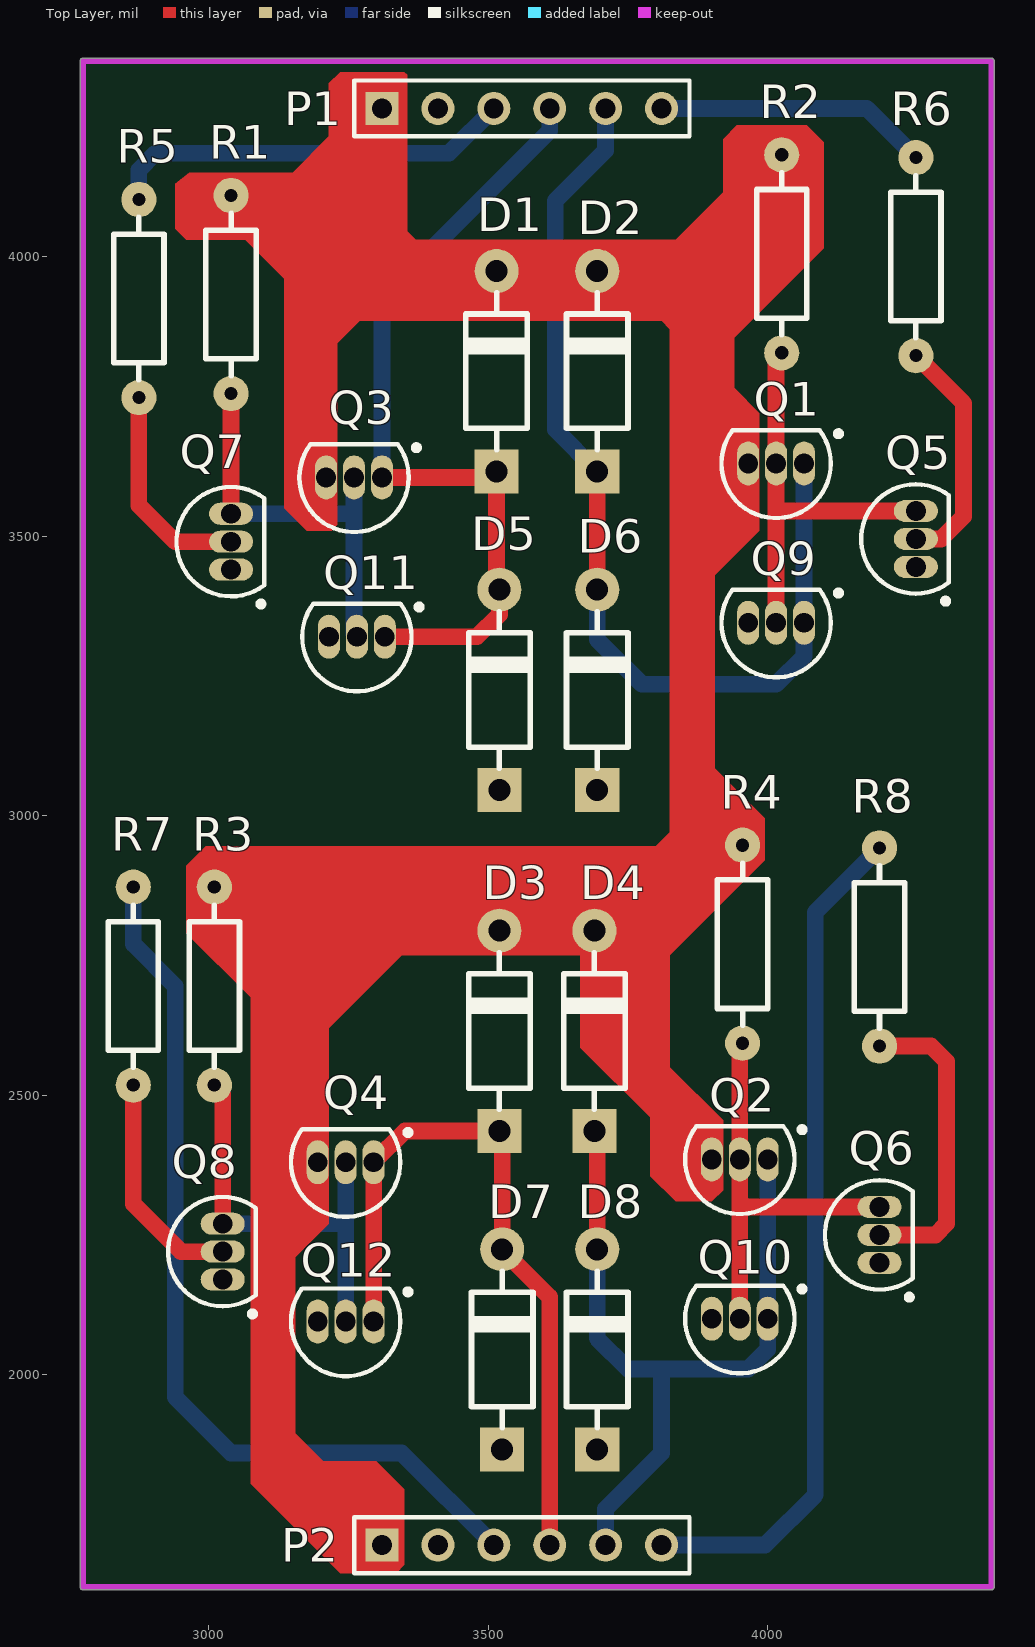
[diagram p0: Top Layer view]
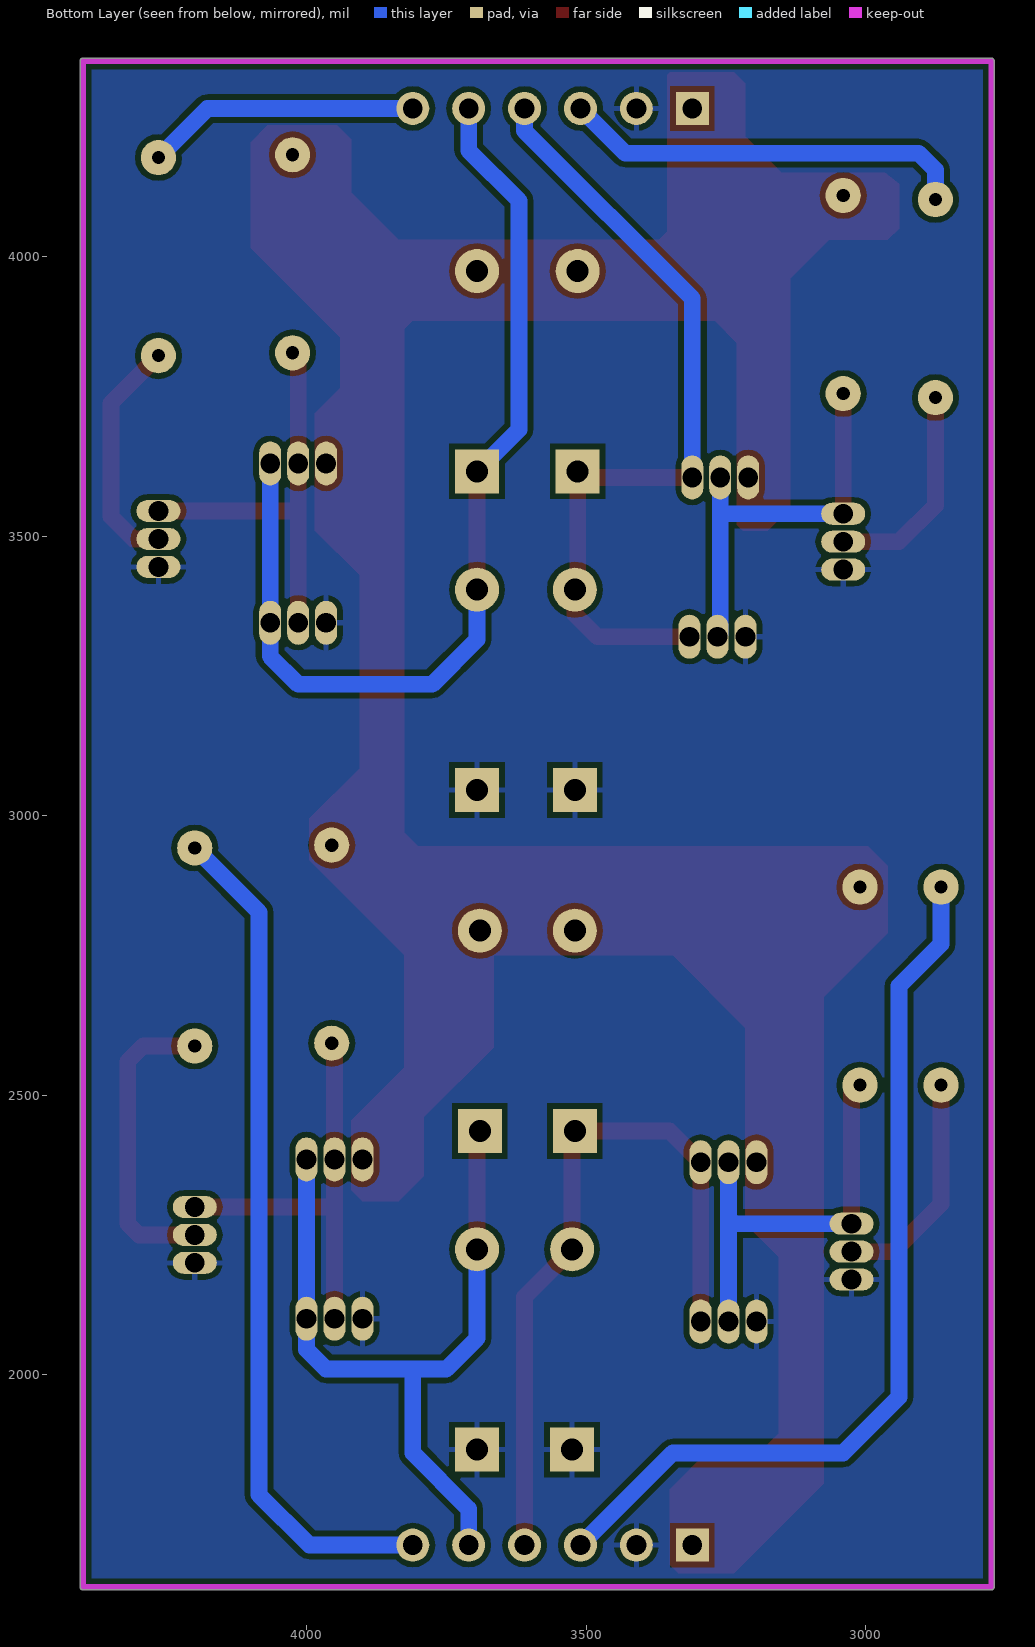
[diagram p1: Bottom Layer view, seen from below]
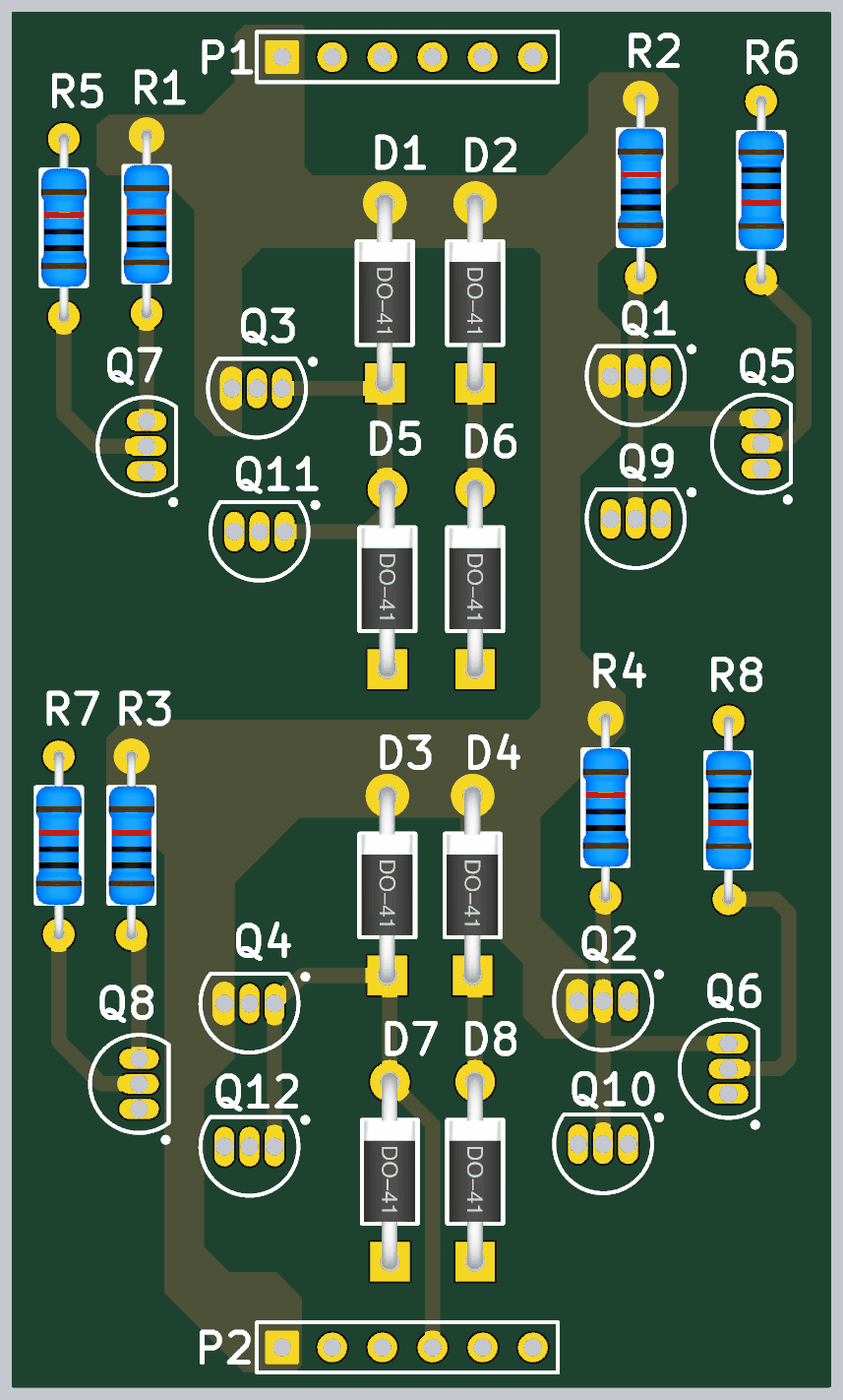
[diagram p2: 3D render of the assembled board from above, using the file's embedded part models]
# Altium PCB MISC84245.PcbDoc
Units mil, origin at the board's own origin, x right, y up, seen from the top; angles counter-clockwise.
Board outline 1635.03 x 2740.03 mil, 2 copper layers (Top Layer, Bottom Layer); 30 components, 18 nets, 80 pads, 0 vias.

## Layer stack, top to bottom (the 12.6 mil dielectric is the usual default, probably not edited)
Top Solder: solder mask 0.4, Solder Resist, Dk 3.5
Top Layer: signal copper 1.4
Dielectric 1: dielectric 12.6, FR-4, Dk 4.8
Bottom Layer: signal copper 1.4
Bottom Solder: solder mask 0.4, Solder Resist, Dk 3.5

## Board outline
2769.99,1620 ccw(c2775,1620) 2775,1614.98 4400,1614.98 ccw(c4400,1620) 4405.02,1620 4405.02,4350 ccw(c4400,4350) 4400,4355.02 2775,4355.02 ccw(c2775,4350) 2769.99,4350

## Design rules (kind name [scope] priority, off if disabled: settings)
Clearance [All] p1: gap=10
MinimumSolderMaskSliver [All] p1: minsoldermaskwidth=0
PolygonConnect [All] p1: connectstyle=Relief reliefconductorwidth=10 reliefentries=4 polygonreliefangle="90 Angle" airgapwidth=10
RoutingVias [All] p1: holewidth=28 width=50 viastyle="Through Hole" minholewidth=28 minwidth=50 maxholewidth=28 maxwidth=50
SilkToSilkClearance [All] p1: silktosilkclearance=0
SilkToSolderMaskClearance [IsPad] p1: minsilkscreentomaskgap=0 clearancetoexposedcopper=TRUE
SolderMaskExpansion [All] p1: expansion=4
Width [All] p1: maxlimit=100 minlimit=10 preferedwidth=10
27 further rules are at their usual default settings.

## Components (designator, comment, footprint, x,y, rotation, side; value= is the part's Value field where it differs from the comment)
D1 "1N4148" DO-41 3515,3795 r90 top
D2 "1N4148" DO-41 3695,3795 r90 top
D3 "1N4148" DO-41 3520,2615 r90 top
D4 "1N4148" DO-41 3690,2615 r90 top
D5 "1N4148" DO-41 3520,3225 r90 top
D6 "1N4148" DO-41 3695,3225 r90 top
D7 "1N4148" DO-41 3525,2045 r90 top
D8 "1N4148" DO-41 3695,2045 r90 top
P1 "Header 6" HDR1X6 3310,4265 r0 top
P2 "Header 6" HDR1X6 3310,1695 r0 top
Q1 "2N3904" TO-92A 4015,3630 r90 top
Q2 "2N3904" TO-92A 3950,2385 r90 top
Q3 "2N3904" TO-92A 3260,3605 r90 top
Q4 "2N3904" TO-92A 3245,2380 r90 top
Q5 "2N3904" TO-92A 4265,3495 r0 top
Q6 "2N3904" TO-92A 4200,2250 r0 top
Q7 "2N3904" TO-92A 3040,3490 r0 top
Q8 "2N3904" TO-92A 3025,2220 r0 top
Q9 "2N3906" TO-92A 4015,3345 r90 top
Q10 "2N3906" TO-92A 3950,2100 r90 top
Q11 "2N3906" TO-92A 3265,3320 r90 top
Q12 "2N3906" TO-92A 3245,2095 r90 top
R1 "1K" "RS 1/4W" 3040,3932.17 r90 top
R2 "1K" "RS 1/4W" 4025,4005 r90 top
R3 "1K" "RS 1/4W" 3010,2695 r90 top
R4 "1K" "RS 1/4W" 3955,2770 r90 top
R5 "100" "RS 1/4W" 2875,3925 r90 top
R6 "100" "RS 1/4W" 4265,4000 r270 top
R7 "100" "RS 1/4W" 2865,2695 r90 top
R8 "100" "RS 1/4W" 4200,2765 r270 top

## Footprints (in the part's own frame and the unit in brackets; to place one, negate y for a bottom-side part, rotate by r counter-clockwise, add the part's x,y. Pads: shape width x height; smd on the part's side, far side on the other; paste and mask are expansions set on the pad)
DO-41 [mm] "2.6*9.1mm(直径，脚距）"
  rect 2x2 hole 1: 1(-4.55,0)
  round 2 hole 1: 2(4.55,0)
  silkscreen extent -3.56,-1.4 3.56,1.4, body extent -4.92,-1.29 4.98,1.31, height 2.65
HDR1X6 [mm] "Connector; Header; 6 Position"
  rect 1.5x1.5 hole 0.9: 1(0,0)
  round 1.5 hole 0.9: 2(2.54,0) 3(5.08,0) 4(7.62,0) 5(10.16,0) 6(12.7,0)
  silkscreen extent -1.27,-1.27 13.97,1.27
"RS 1/4W" [mm] "直插色环电阻，脚距9mm，直径2.3mm"
  round 1.6 hole 0.6: 1(-4.5,0) 2(4.5,0)
  silkscreen extent -3.68,-1.14 3.68,1.14, body extent -4.72,-1.16 4.73,1.16, height 2.32
TO-92A [mm] "TO, Flat Index; 3 In-Line, Axial Leads; Body Dia. 4.5mm; Leads 0.51 x 0.48 mm (max)"
  oval 2x1 hole 0.9: 1(0,-1.27) 2(0,0) 3(0,1.27)
  silkscreen extent -2.48,-2.96 1.5,2.48, body extent -2.48,-2.5 1.5,2.5, height 6.86

## Part data
D1 D2 D3 D4 D5 D6 D7 D8: "Switching diode"
P1 P2: "Header, 6-Pin"
Q1 Q2 Q3 Q4 Q5 Q6 Q7 Q8: "NPN General Purpose Amplifier"
Q9 Q10 Q11 Q12: "PNP General Purpose Amplifier"
R1 R2 R3 R4 R5 R6 R7 R8: library part R-S, "Color-band resistor"

## Nets (pads, with @x,y where several pads share a name; then routed paths per layer and width w, separated by ;. In a path a pad name is that pad's centre, name@x,y a point inside that pad or via, vN(x,y) a via of type N, cw(c..) or ccw(c..) an arc to the next point about the centre after c; other vN are vias at no path point)
A: P1.3 R5.2 | length 733.4
  Bottom Layer w30: R5.2 2875,4155 2905,4185 3430,4185 P1.3
B: D1.1 D5.2 P1.4 Q3.1 Q11.1 | length 1473.3
  Top Layer w30: Q3.1 3504.13,3605 D1.1 3515,3409.13 D5.2 3520,3360 3480,3320 Q11.1
  Bottom Layer w30: Q3.1 3310,3925 3610,4225 P1.4
C: D2.1 D6.2 P1.5 Q1.1 Q9.1 | length 1787.2
  Top Layer w30: D6.2 D2.1
  Bottom Layer w30: D6.2 3695,3315 3775,3235 4015,3235 4065,3285 Q9.1 Q1.1 ; D2.1 3620,3690.87 3620,4100 3710,4190 P1.5
D: P1.6 R6.1 | length 491.4
  Bottom Layer w30: P1.6 4177.17,4265 R6.1
E: P2.3 R7.2 | length 1623
  Bottom Layer w30: R7.2 2865,2770 2940,2695 2940,1960 3040,1860 3345,1860 P2.3
F: D3.1 D7.2 P2.4 Q4.1 Q12.1 | length 1311.3
  Top Layer w30: Q12.1 Q4.1 3350.87,2435.87 D3.1 3525,2430.87 D7.2 3610,2139.13 P2.4
G: D4.1 D8.2 P2.5 Q2.1 Q10.1 | length 1411.6
  Top Layer w30: D4.1 3695,2430.87 D8.2
  Bottom Layer w30: D8.2 3695,2065 3750,2010 3810,2010 ; P2.5 3710,1760 3810,1860 3810,2010 ; Q2.1 Q10.1 4000,2045 3965,2010 3810,2010
GND: D5.1 D6.1 D7.1 D8.1 P1.2 P2.2 Q5.1 Q6.1 Q7.1 Q8.1 Q9.3 Q10.3 Q11.3 Q12.3
H: P2.6 R8.1 | length 1517.1
  Bottom Layer w30: P2.6 3995,1695 4085,1785 4085,2827.17 R8.1
NetQ1_2: Q1.2 Q5.3 Q9.2 R2.1 | length 737
  Top Layer w30: Q9.2 4015,3545 ; R2.1 4015,3817.83 Q1.2 4015,3545 ; Q5.3 4015,3545
NetQ2_2: Q2.2 Q6.3 Q10.2 R4.1 | length 749
  Top Layer w30: Q10.2 3950,2310 ; R4.1 3950,2587.83 Q2.2 3950,2310 ; Q6.3 3960,2300 3950,2310
NetQ3_2: Q3.2 Q7.3 Q11.2 R1.1 | length 724.1
  Top Layer w30: Q7.3 R1.1
  Bottom Layer w30: Q7.3 3255,3540 3260,3535 ; Q3.2 3260,3535 ; Q11.2 3260,3325 3260,3535
NetQ4_2: Q4.2 Q8.3 Q12.2 R3.1 | length 763.2
  Top Layer w30: R3.1 3025,2502.83 Q8.3
  Bottom Layer w30: Q8.3 3235,2270 3245,2280 ; Q12.2 3245,2280 ; Q4.2 3245,2280
NetQ5_2: Q5.2 R6.2 | length 424.6
  Top Layer w30: Q5.2 4310,3495 4350,3535 4350,3737.83 R6.2
NetQ6_2: Q6.2 R8.2 | length 549.8
  Top Layer w30: Q6.2 4300,2250 4320,2270 4320,2560 4292.17,2587.83 R8.2
NetQ7_2: Q7.2 R5.1 | length 384.8
  Top Layer w30: R5.1 2875,3555 2940,3490 Q7.2
NetQ8_2: Q8.2 R7.1 | length 408
  Top Layer w30: R7.1 2865,2305 2950,2220 Q8.2
VCC: D1.2 D2.2 D3.2 D4.2 P1.1 P2.1 Q1.3 Q2.3 Q3.3 Q4.3 R1.2 R2.2 R3.2 R4.2

## Polygon pours and split planes (outlines as drawn)
GND on Bottom Layer "D" (solid, remove dead copper, pour order 0): 2445,4490 2500,4545 4525,4545 4525,1475 4480,1430 4410,1360 2595,1360

## Keep-outs
Keep-Out Layer:
  lines w10: 3200,4350 4400,4350 4400,1620 2850,1620 2775,1620 2775,4350 2785,4350 3210,4350

## Other copper
Top Layer:
  region net VCC: 3825,2750 3825,2550 3920,2455 3920,2330 3900,2310 3835,2310 3790,2355 3790,2460 3665,2585 3665,2750
  region net VCC: 2965,4150 3150,4150 3215,4215 3215,4310 3235,4330 3350,4330 3355,4325 3355,4045 3370,4030 3565,4030 3835,4030 3920,4115 3920,4210 3945,4235 4070,4235 4100,4205 4100,4015 3940,3855 3940,3765 3985,3720 3985,3510 3905,3430 3905,3085 3995,2995 3995,2920 3825,2750 3345,2750 3215,2620 3215,2270 3155,2210 3155,1895 3205,1845 3300,1845 3350,1795 3350,1660 3335,1645 3235,1645 3075,1805 3075,2410 3075,2675 2960,2790 2960,2910 2995,2945 3800,2945 3825,2970 3825,3665 3825,3870 3810,3885 3270,3885 3230,3845 3230,3520 3220,3510 3175,3510 3135,3550 3135,3960 3065,4030 2960,4030 2940,4050 2940,4130